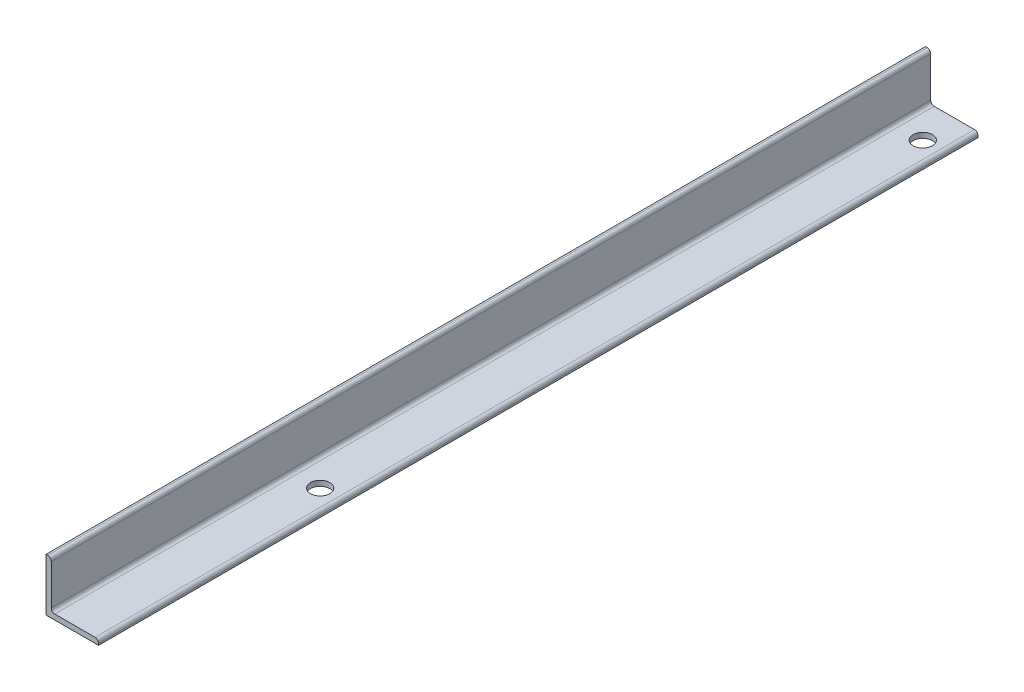
SolidWorks part; units mm, degrees
material "Plain Carbon Steel"
ref_plane "Front Plane" through (0, 0, 0) normal (0, 0, 1) x (1, 0, 0)
ref_plane "Top Plane" through (0, 0, 0) normal (0, 1, 0) x (1, 0, 0)
ref_plane "Right Plane" through (0, 0, 0) normal (1, 0, 0) x (0, 0, -1)
sketch "Sketch1" plane through (0, 0, 0) normal (0, 0, 1) x (1, 0, 0)
  line L0 (0, 0) -> (30, 0)
  line L1 (0, 0) -> (0, 30)
  line L2 (5, 3) -> (28, 3)
  line L3 (3, 5) -> (3, 28)
  line L4 (0, 30) -> (1, 30)
  line L5 (30, 1) -> (30, 0)
  line L6 (3, 3) -> (3, 30) construction
  line L7 (3, 3) -> (30, 3) construction
  arc A0 (1, 30) -> (3, 28) centre (1, 28) cw
  arc A1 (5, 3) -> (3, 5) centre (5, 5) cw
  arc A2 (30, 1) -> (28, 3) centre (28, 1) ccw
  dimension "D3" = 2
  dimension "D1" = 30
  dimension "D2" = 3
extrude "Boss-Extrude1" add sketch "Sketch1" along normal blind 502
sketch "Sketch2" plane through (0, 0, 0) normal (0, -1, 0) x (1, 0, 0)
  line L1 (0, 502) -> (0, 0) construction
  line L2 (0, 0) -> (30, 0) construction
  circle A0 centre (18.5, 20) radius 5.5
  dimension "D3" = 11
  dimension "D1" = 20
  dimension "D2" = 18.5
extrude "Cut-Extrude1" cut sketch "Sketch2" against normal blind 3
pattern_linear "LPattern1" count 2 spacing 344 along (0, 0, 1) of "Cut-Extrude1"
